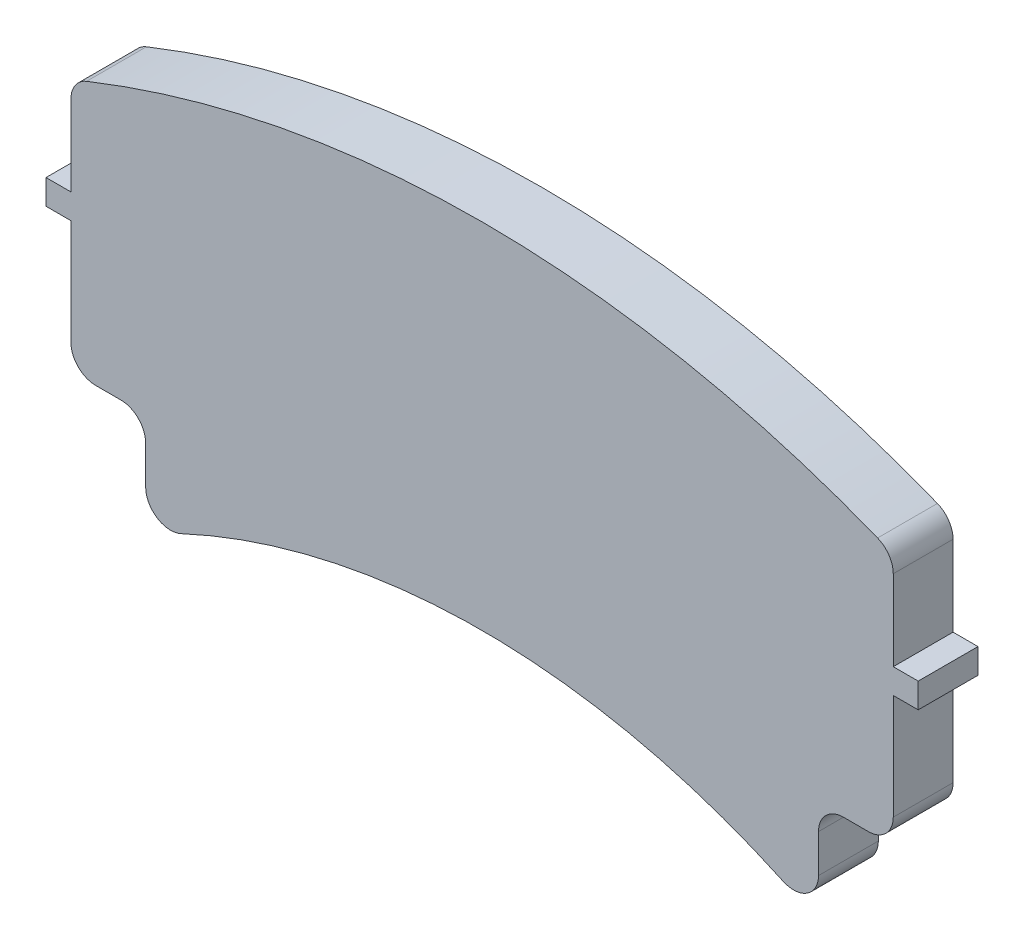
SolidWorks part; units mm, degrees
ref_plane "Front Plane" through (0, 0, 0) normal (0, 0, 1) x (1, 0, 0)
ref_plane "Top Plane" through (0, 0, 0) normal (0, 1, 0) x (1, 0, 0)
ref_plane "Right Plane" through (0, 0, 0) normal (1, 0, 0) x (0, 0, -1)
sketch "Sketch1" plane through (0, 0, 0) normal (0, 0, 1) x (1, 0, 0)
  line L0 (-82.5, 197.4582) -> (-82.5, 116.8022)
  line L1 (82.5, 197.4582) -> (82.5, 116.8022)
  arc A0 (82.5, 197.4582) -> (-82.5, 197.4582) centre (0, 0) ccw
  arc A1 (82.5, 116.8022) -> (-82.5, 116.8022) centre (0, 0) ccw
  dimension "D1" = 286
  dimension "D2" = 428
  dimension "D3" = 165
  dimension "D4" = 82.5
extrude "Boss-Extrude1" add sketch "Sketch1" along normal mid plane 12
sketch "Sketch2" plane through (0, 0, 6) normal (0, 0, 1) x (1, 0, 0)
  line L0 (0, 0) -> (0, 41.5109) construction
  line L1 (-82.5, 116.8022) -> (-67.5, 116.8022)
  line L2 (-82.5, 116.8022) -> (-82.5, 146.8022)
  line L3 (-82.5, 146.8022) -> (-67.5, 146.8022)
  line L4 (-67.5, 116.8022) -> (-67.5, 146.8022)
  line L5 (82.5, 146.8022) -> (67.5, 146.8022)
  line L6 (67.5, 116.8022) -> (67.5, 146.8022)
  line L7 (82.5, 116.8022) -> (67.5, 116.8022)
  line L8 (82.5, 116.8022) -> (82.5, 146.8022)
  arc A0 (82.5, 116.8022) -> (-82.5, 116.8022) centre (0, 0) ccw construction
  dimension "D1" = 30
  dimension "D2" = 15
extrude "Cut-Extrude1" cut sketch "Sketch2" against normal blind 30
fillet "Fillet2" radius 5 8 edges at (82.5, 197.4582, 0) (82.5, 146.8022, 0) (67.5, 146.8022, 0) (67.5, 126.0665, 0) (-67.5, 126.0665, 0) (-67.5, 146.8022, 0) (-82.5, 146.8022, 0) (-82.5, 197.4582, 0)
sketch "Sketch3" plane through (0, 0, 6) normal (0, 0, 1) x (1, 0, 0)
  line L0 (82.5, 151.8022) -> (82.5, 194.0998) construction
  line L1 (82.5, 172.951) -> (87.5, 172.951)
  line L2 (82.5, 172.951) -> (82.5, 177.951)
  line L3 (82.5, 177.951) -> (87.5, 177.951)
  line L4 (87.5, 172.951) -> (87.5, 177.951)
  line L5 (0, 0) -> (0, 51.0012) construction
  line L6 (-82.5, 177.951) -> (-87.5, 177.951)
  line L7 (-87.5, 172.951) -> (-87.5, 177.951)
  line L8 (-82.5, 172.951) -> (-87.5, 172.951)
  line L9 (-82.5, 172.951) -> (-82.5, 177.951)
  dimension "D1" = 5
extrude "Boss-Extrude2" add sketch "Sketch3" against normal up to surface (12 mm away) up to face at (0, 157.085, -6)
